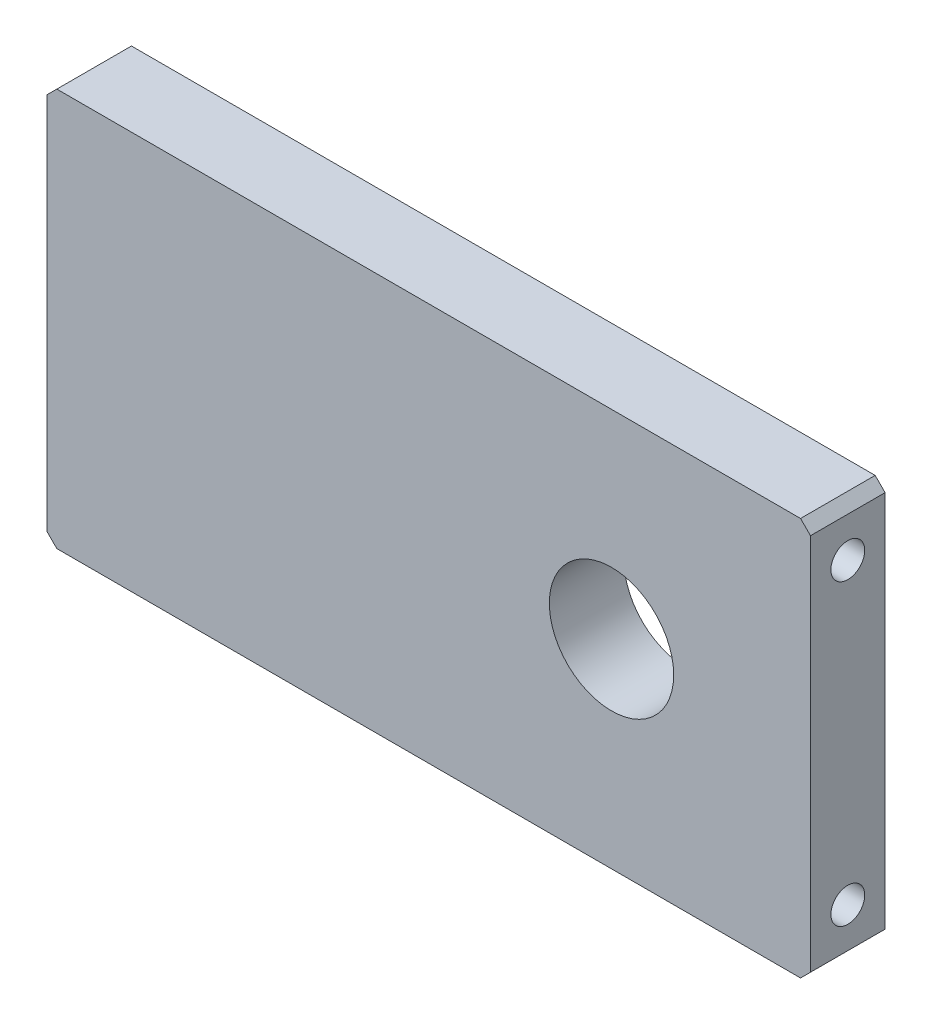
SolidWorks part; units mm, degrees
ref_plane "前视基准面" through (0, 0, 0) normal (0, 0, 1) x (1, 0, 0)
ref_plane "上视基准面" through (0, 0, 0) normal (0, 1, 0) x (1, 0, 0)
ref_plane "右视基准面" through (0, 0, 0) normal (1, 0, 0) x (0, 0, -1)
sketch "草图1" plane through (0, 0, 0) normal (0, 0, 1) x (1, 0, 0)
  line L1 (-76.75, 40) -> (76.75, 40)
  line L2 (-76.75, 40) -> (-76.75, -40)
  line L3 (-76.75, -40) -> (76.75, -40)
  line L4 (76.75, 40) -> (76.75, -40)
  line L5 (-76.75, 40) -> (76.75, -40) construction
  line L6 (-76.75, -40) -> (76.75, 40) construction
  point P0 (0, 0)
  dimension "D1" = 153.5
  dimension "D2" = 80
extrude "凸台-拉伸1" add sketch "草图1" along normal mid plane 15
hole_wizard "Ø25.0 (25) 直径孔1" positions "草图3" profile "草图2" hole size "Ø25.0" standard "ISO" end condition through all
sketch "草图3" plane through (0, 0, 7.5) normal (0, 0, 1) x (1, 0, 0)
  line L0 (76.75, -40) -> (76.75, 40) construction
  line L1 (-76.75, -40) -> (76.75, -40) construction
  point P0 (36.75, 0)
  dimension "D1" = 40
  dimension "D2" = 40
sketch "草图2" plane through (36.75, 0, 7.5) normal (1, 0, 0) x (0, -1, 0)
  line L0 (0, 0) -> (0, 15)
  line L1 (0, 15) -> (12.5, 15)
  line L2 (12.5, 15) -> (12.5, 0)
  line L5 (12.5, 0) -> (0, 0)
  line L11 (0, -6.35) -> (0, 107.95) construction
  dimension "通孔孔直径" = 25
  dimension "通孔孔深度" = 15
hole_wizard "M8 螺纹孔1" positions "草图5" profile "草图4" tap size "M8" standard "ISO"
sketch "草图5" plane through (76.75, 0, 0) normal (1, 0, 0) x (0, 0, -1)
  line L0 (-7.5, -40) -> (7.5, -40) construction
  point P0 (0, -30)
  point P2 (0, 30)
  dimension "D1" = 60
  dimension "D2" = 10
sketch "草图4" plane through (76.75, -30, 0) normal (0, 1, 0) x (0, 0, -1)
  line L0 (0, 0) -> (0, 21.7929)
  line L1 (0, 21.7929) -> (3.4, 19.75)
  line L2 (3.4, 19.75) -> (3.4, 0)
  line L5 (3.4, 0) -> (0, 0)
  line L10 (0, 21.7929) -> (-3.4, 19.75) construction
  line L11 (0, -6.35) -> (0, 107.95) construction
  dimension "螺纹孔钻头直径" = 6.8
  dimension "螺纹孔钻头深度" = 19.75
  dimension "导头角度" = 118
cosmetic thread "孔螺蚊线1" parameters "D1"=16, "D2"=8
cosmetic thread "孔螺蚊线2" parameters "D1"=16, "D2"=8
mirror "镜向1" about plane through (0, 0, 0) normal (1, 0, 0) of "M8 螺纹孔1"
sketch "草图6" plane through (-76.75, 0, 0) normal (-1, 0, 0) x (0, 0, 1)
  line L0 (-52.5, 14.2972) -> (-52.5, -19.1842) construction
  line L1 (12.2176, 0) -> (-55.0572, 0) construction
  line L3 (-7.5, 40) -> (-7.5, -40) construction
  circle A0 centre (-52.5, 0) radius 56
  dimension "D2" = 112
  dimension "D1" = 45
extrude "切除-拉伸1" cut sketch "草图6" against normal blind 10
chamfer "倒角1" distance 2 angle 45 4 edges at (76.75, 40, 0) (76.75, -40, 0) (-76.75, -40, 0) (-76.75, 40, 0)
